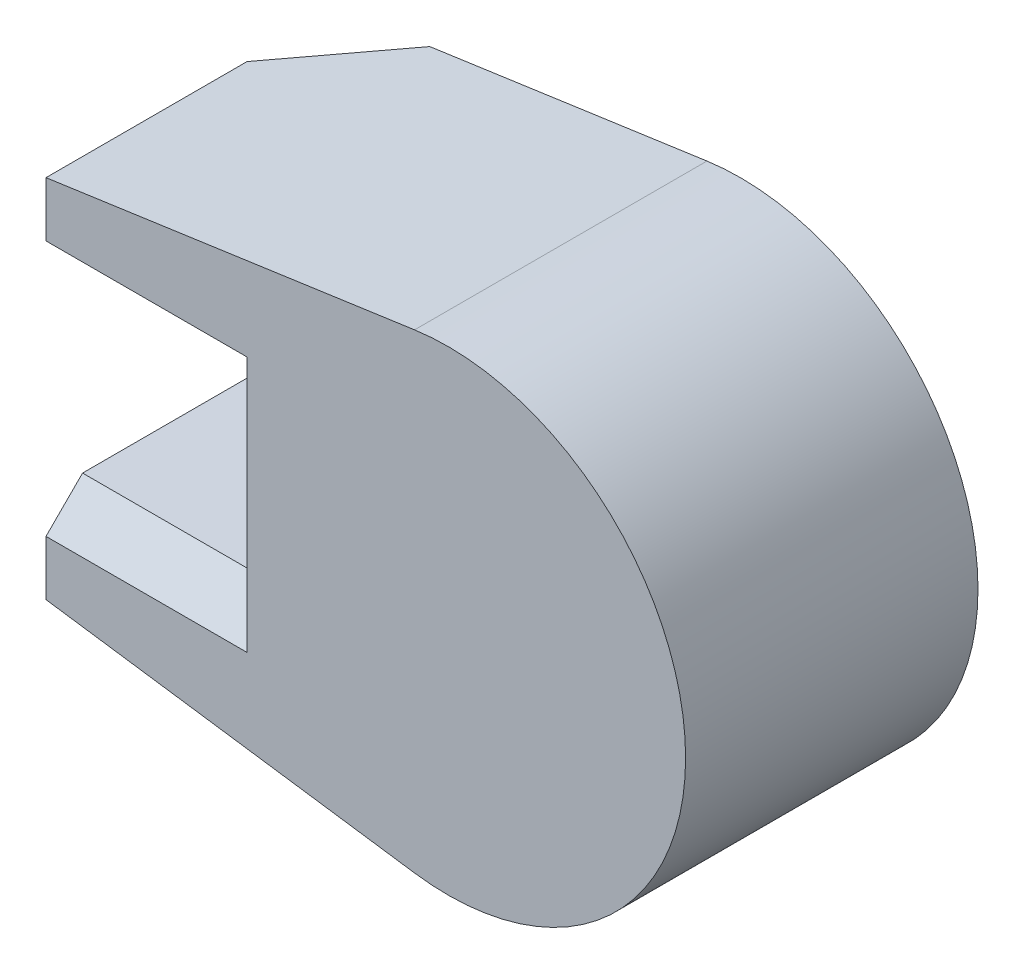
SolidWorks part; units mm, degrees
material "普通碳钢"
ref_plane "前视" through (0, 0, 0) normal (0, 0, 1) x (1, 0, 0)
ref_plane "上视" through (0, 0, 0) normal (0, 1, 0) x (1, 0, 0)
ref_plane "右视" through (0, 0, 0) normal (1, 0, 0) x (0, 0, -1)
sketch "草图1" plane through (0, 0, 0) normal (0, 0, 1) x (1, 0, 0)
  line L0 (-112.3085, 0) -> (100.0953, 0) construction
  line L1 (0, 82.1737) -> (0, -83.5012) construction
  line L2 (-110, 50) -> (-110, 25)
  line L3 (-110, 50) -> (-9.1584, 64.3516)
  line L4 (-110, -50) -> (-9.1584, -64.3516)
  line L5 (-110, 25) -> (-65, 25)
  line L6 (-65, 25) -> (-65, -25)
  line L7 (-65, -25) -> (-110, -25)
  line L8 (-110, -25) -> (-110, -50)
  arc A0 (-9.1584, -64.3516) -> (-9.1584, 64.3516) centre (0, 0) ccw
  dimension "D1" = 130
  dimension "D2" = 110
  dimension "D3" = 100
  dimension "D4" = 50
  dimension "D5" = 45
extrude "凸台-拉伸1" add sketch "草图1" along normal mid plane 80
chamfer "倒角1" distance 25 angle 45 2 edges at (-110, -37.5, -40) (-110, 37.5, -40)
chamfer "倒角2" distance 10 angle 45 3 edges at (-87.5, -25, 40) (-65, 0, 40) (-87.5, 25, 40)
chamfer "倒角3" distance 10 angle 45 3 edges at (-75, -25, -40) (-65, 0, -40) (-75, 25, -40)
